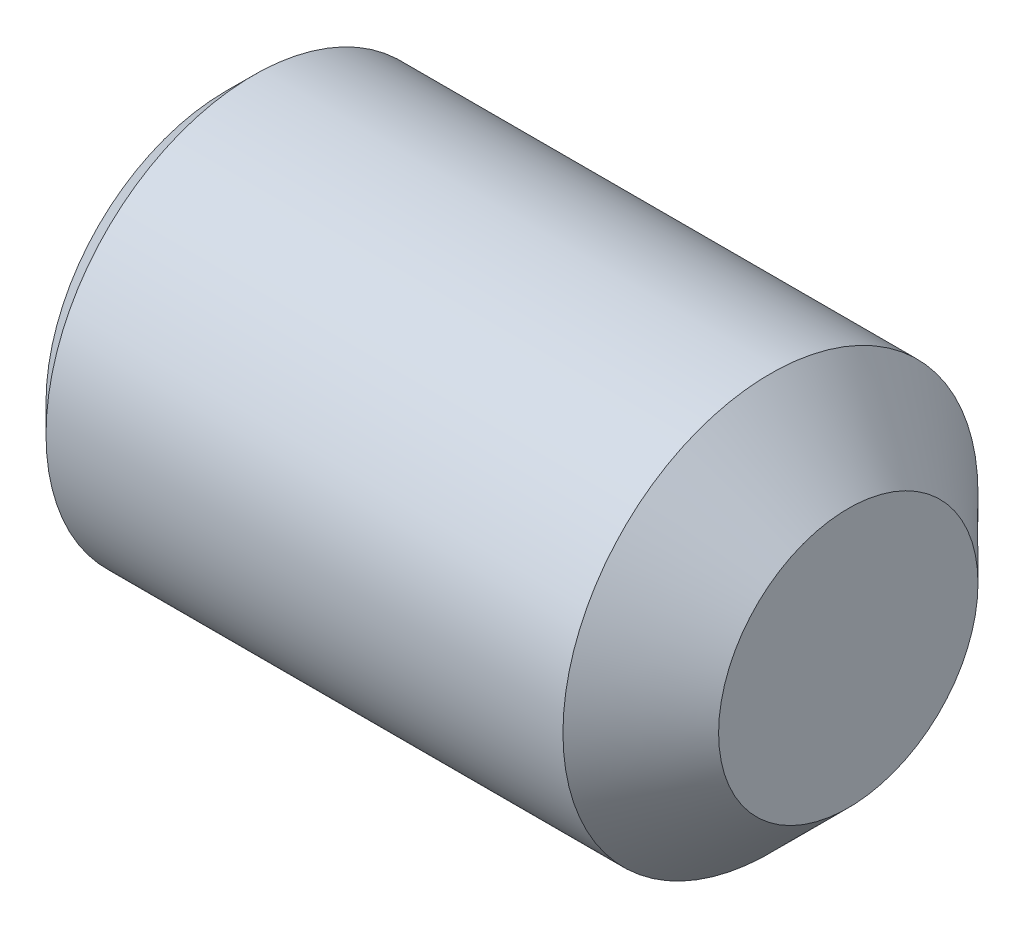
SolidWorks part; units mm, degrees
revolve "Boss-Revolve" add sketch "Sketch1" angle 360 about L6
sketch "Sketch1" plane through (0, 0, 0) normal (0, 0, 1) x (1, 0, 0)
  line L0 (0, 0) -> (6, 0)
  line L1 (6, 0) -> (6, 1.25)
  line L2 (6, 1.25) -> (5.25, 2)
  line L3 (5.25, 2) -> (0.268, 2)
  line L4 (0.268, 2) -> (0, 1.732)
  line L5 (0, 1.732) -> (0, 0)
  line L6 (-0.2778, 0) -> (5.1995, 0) construction
cosmetic thread "Cosmetic Thread1" parameters "df"=3.464
extrude "Cut-Extrude1" cut sketch "Sketch2" against normal blind 1.5
sketch "Sketch2" plane through (0, 0, 0) normal (-1, 0, 0) x (0, 0, 1)
  line L1 (-0.575, -0.9959) -> (0.575, -0.9959)
  line L2 (0.575, -0.9959) -> (1.15, 0)
  line L3 (1.15, 0) -> (0.575, 0.9959)
  line L4 (0.575, 0.9959) -> (-0.575, 0.9959)
  line L5 (-0.575, 0.9959) -> (-1.15, 0)
  line L6 (-1.15, 0) -> (-0.575, -0.9959)
  circle A0 centre (0, 0) radius 0.9959 construction
material "Grade 45H"
ref_plane "Front" through (0, 0, 0) normal (0, 0, 1) x (1, 0, 0)
ref_plane "Top" through (0, 0, 0) normal (0, 1, 0) x (1, 0, 0)
ref_plane "Right" through (0, 0, 0) normal (1, 0, 0) x (0, 0, -1)
sketch "Dimension Sketch" plane through (0, 0, 0) normal (0, 0, 1) x (1, 0, 0)
  line L0 (0, 0) -> (6, 0)
  point P3 (1.5, 0)
  point P4 (5.3, 0)
  point P5 (3.5, 0)
  point P6 (3.464, 0)
  point P7 (4, 0)
  point P8 (3.7, 0)
sketch "Sketch4" plane through (0, 0, 0) normal (0, 0, 1) x (1, 0, 0)
  line L0 (-0.2778, 0) -> (1.1933, 0) construction
  line L2 (-0.2778, 0) -> (5.1995, 0) construction
  line L3 (1.5, 0.9959) -> (2.075, 0)
  line L4 (2.075, 0) -> (1.5, 0)
  line L5 (1.5, 0) -> (1.5, 0.9959)
  line L6 (1.5, 0.9959) -> (0, 0.9959) construction
revolve "Cut-Revolve2" cut sketch "Sketch4" angle 360 about L0
sketch "Sketch5" plane through (0, 0, 0) normal (0, 0, 1) x (1, 0, 0)
  line L0 (0.268, 2) -> (0.968, 2)
  line L1 (5.25, 2) -> (0.268, 2) construction
  line L2 (0.968, 2) -> (0.6142, 1.3938)
  line L3 (0.6142, 1.3938) -> (0.268, 2)
  line L5 (5.1995, 0) -> (3.6008, 0) construction
  line L6 (-0.2778, 0) -> (5.1995, 0) construction
  line L7 (0.268, 2) -> (0, 1.732) construction
revolve "Cut-Revolve3" [suppressed] cut sketch "Sketch5" angle 360 about L5
pattern_linear "LPattern1" [suppressed] count 9
equation "\"l@Sketch1\"=\"l@Dimension Sketch\""
equation "\"d@Sketch1\"=\"d@Dimension Sketch\""
equation "\"df@Sketch1\" = \"df@Dimension Sketch\""
equation "\"dp@Sketch1\" = \"dp@Dimension Sketch\""
equation "\"e@Sketch2\" = \"e@Dimension Sketch\""
equation "\"t@Cut-Extrude1\" = \"t@Dimension Sketch\""
equation "\"P@Sketch5\" = \"P@Dimension Sketch\""
equation "\"D1@Sketch5\" = \"P@Dimension Sketch\"*0.866"
equation "\"P@LPattern1\" = \"P@Dimension Sketch\""
equation "\"D1@LPattern1\" = \"l@Dimension Sketch\"/\"P@Dimension Sketch\""
equation "\"df@Cosmetic Thread1\"=\"df@Dimension Sketch\""
equation "\"D2@Sketch4\" = \"t@Dimension Sketch\""
